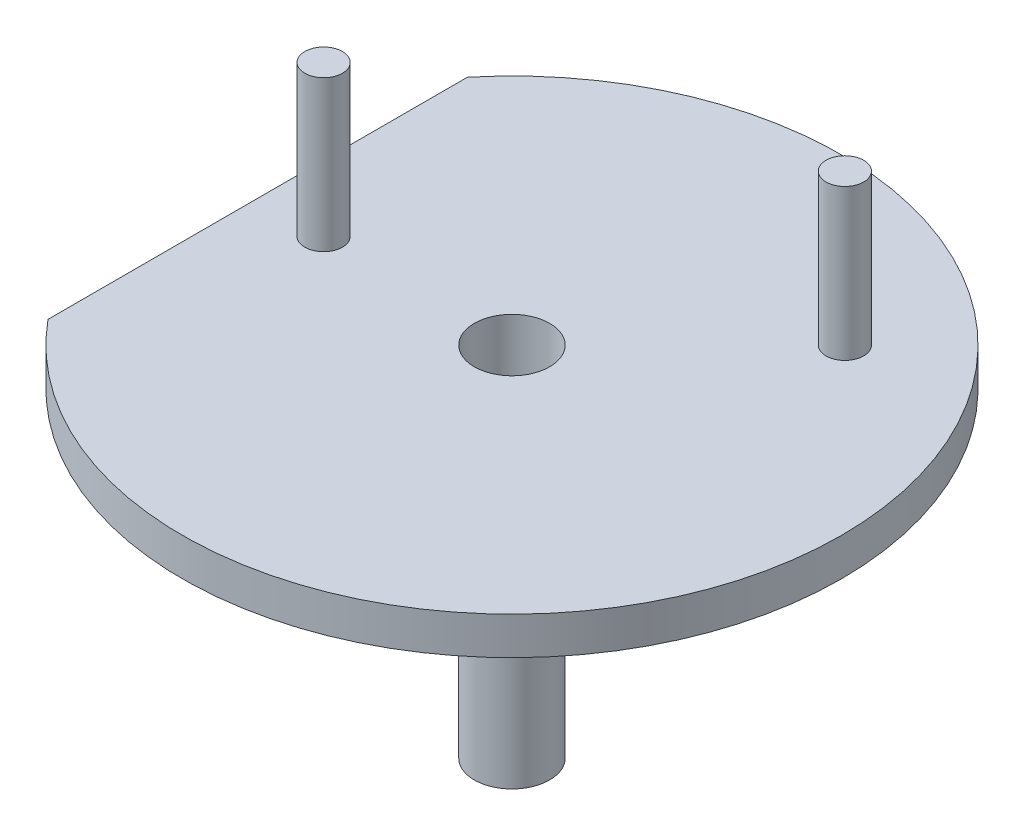
SolidWorks part; units mm, degrees
ref_plane "Front Plane" through (0, 0, 0) normal (0, 0, 1) x (1, 0, 0)
ref_plane "Top Plane" through (0, 0, 0) normal (0, 1, 0) x (1, 0, 0)
ref_plane "Right Plane" through (0, 0, 0) normal (1, 0, 0) x (0, 0, -1)
other "Configuration Table"
sketch "Sketch1" plane through (0, 0, 0) normal (0, 1, 0) x (1, 0, 0)
  circle A0 centre (0, 0) radius 17.5
  dimension "D1" = 35
extrude "Boss-Extrude1" add sketch "Sketch1" along normal blind 2
sketch "Sketch3" plane through (0, 0, 0) normal (0, -1, 0) x (1, 0, 0)
  circle A0 centre (0, 0) radius 4
  dimension "D1" = 8
extrude "Boss-Extrude2" add sketch "Sketch3" along normal blind 2
chamfer "Chamfer1" distance 1 angle 45 1 edges at (0, 0, -4)
sketch "Sketch4" plane through (0, -2, 0) normal (0, -1, 0) x (1, 0, 0)
  circle A0 centre (0, 0) radius 2
  dimension "D1" = 4
extrude "Boss-Extrude3" add sketch "Sketch4" along normal blind 15
sketch "Sketch5" plane through (0, -17, 0) normal (0, -1, 0) x (1, 0, 0)
  circle A0 centre (0, 0) radius 1.5
  dimension "D1" = 3
extrude "Cut-Extrude1" cut sketch "Sketch5" against normal up to surface (15 mm away) up to face at (0, -2, -2)
sketch "Sketch6" plane through (0, 2, 0) normal (0, 1, 0) x (1, 0, 0)
  line L0 (0, 0) -> (0, -50000) construction
  line L1 (0, 0) -> (-50000, 0) construction
  line L2 (0, 0) -> (35355.3391, 35355.3391) construction
  circle A0 centre (0, 0) radius 12.5 construction
  circle A6 centre (0, 0) radius 10 construction
  circle A9 centre (-10, 0) radius 1
  circle A10 centre (8.8388, 8.8388) radius 1
  dimension "D1" = 25
  dimension "D2" = 20
  dimension "D3" = 2
  dimension "D4" = 45
  dimension "D5" = 2
extrude "Boss-Extrude4" add sketch "Sketch6" along normal blind 8
sketch "Sketch7" plane through (0, 2, 0) normal (0, 1, 0) x (1, 0, 0)
  line L0 (0, 0) -> (-50000, 0) construction
  line L1 (0, 0) -> (0, 50000) construction
  line L2 (-17.5, -22.8036) -> (-17.5, 22.8036)
  line L3 (-17.5, 22.8036) -> (-13.5, 22.8036)
  line L4 (-13.5, 22.8036) -> (-13.5, -22.8036)
  line L5 (-17.5, -22.8036) -> (-13.5, -22.8036)
  circle A0 centre (0, 0) radius 17.5 construction
  point P11 (-17.5, 0)
  point P13 (-13.5, 0)
  dimension "D1" = 4
extrude "Cut-Extrude2" cut sketch "Sketch7" against normal through all
sketch "Sketch8" plane through (0, 2, 0) normal (0, 1, 0) x (1, 0, 0)
  circle A0 centre (0, 0) radius 2
  dimension "D1" = 4
extrude "Cut-Extrude3" cut sketch "Sketch8" against normal blind 3
